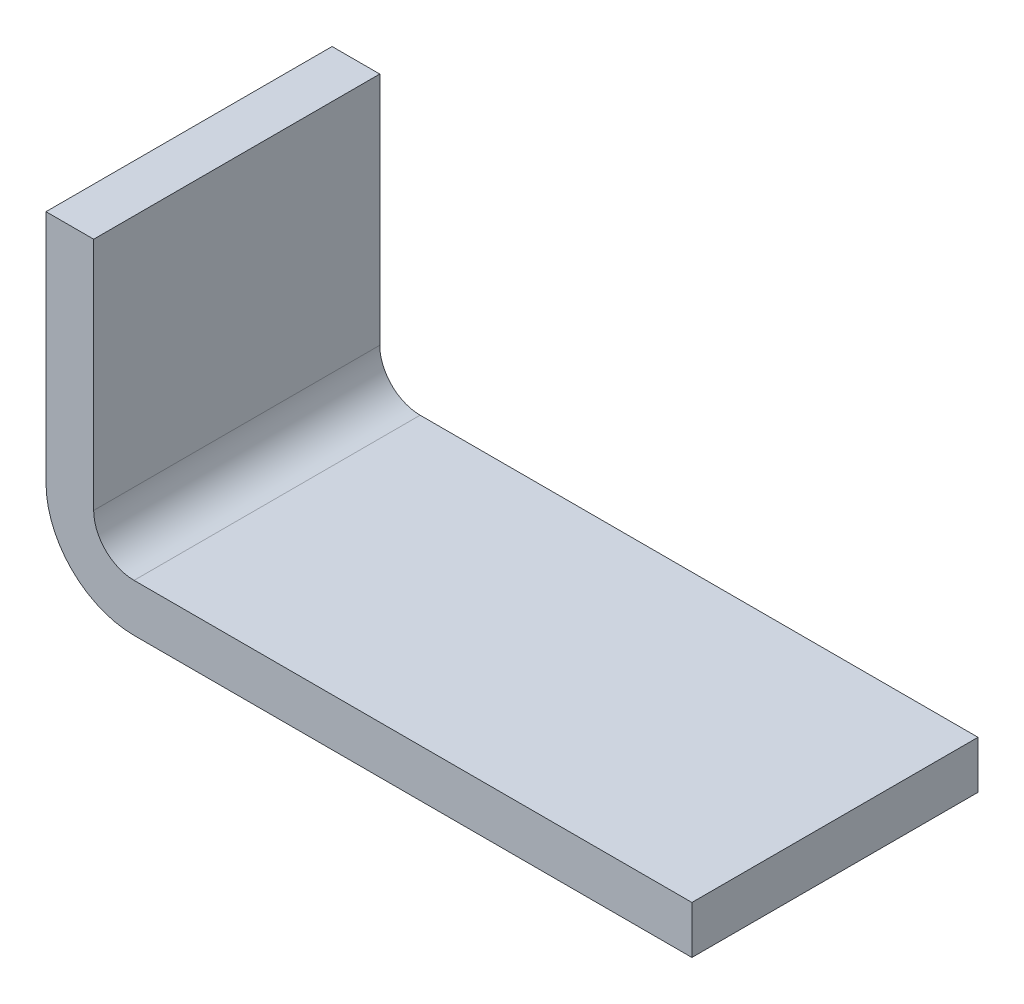
SolidWorks part; units mm, degrees
ref_plane "Front Plane" through (0, 0, 0) normal (0, 0, 1) x (1, 0, 0)
ref_plane "Top Plane" through (0, 0, 0) normal (0, 1, 0) x (1, 0, 0)
ref_plane "Right Plane" through (0, 0, 0) normal (1, 0, 0) x (0, 0, -1)
sketch "Sketch1" plane through (0, 0, 0) normal (0, 0, 1) x (1, 0, 0)
  line L0 (-23.9529, 5.3561) -> (-23.9529, -31.5939)
  line L1 (-10.1029, -45.4439) -> (77.6471, -45.4439)
  line L2 (77.6471, -45.4439) -> (77.6471, -37.9439)
  line L3 (77.6471, -37.9439) -> (-10.1029, -37.9439)
  line L4 (-16.4529, -31.5939) -> (-16.4529, 5.3561)
  line L5 (-16.4529, 5.3561) -> (-23.9529, 5.3561)
  arc A0 (-10.1029, -37.9439) -> (-16.4529, -31.5939) centre (-10.1029, -31.5939) cw
  arc A1 (-23.9529, -31.5939) -> (-10.1029, -45.4439) centre (-10.1029, -31.5939) ccw
  point P10 (-23.9529, -45.4439)
  dimension "D5" = 6.35
  dimension "D6" = 13.85
  dimension "D1" = 7.5
  dimension "D2" = 7.5
  dimension "D3" = 101.6
  dimension "D4" = 50.8
extrude "Extrude1" add sketch "Sketch1" along normal blind 45
